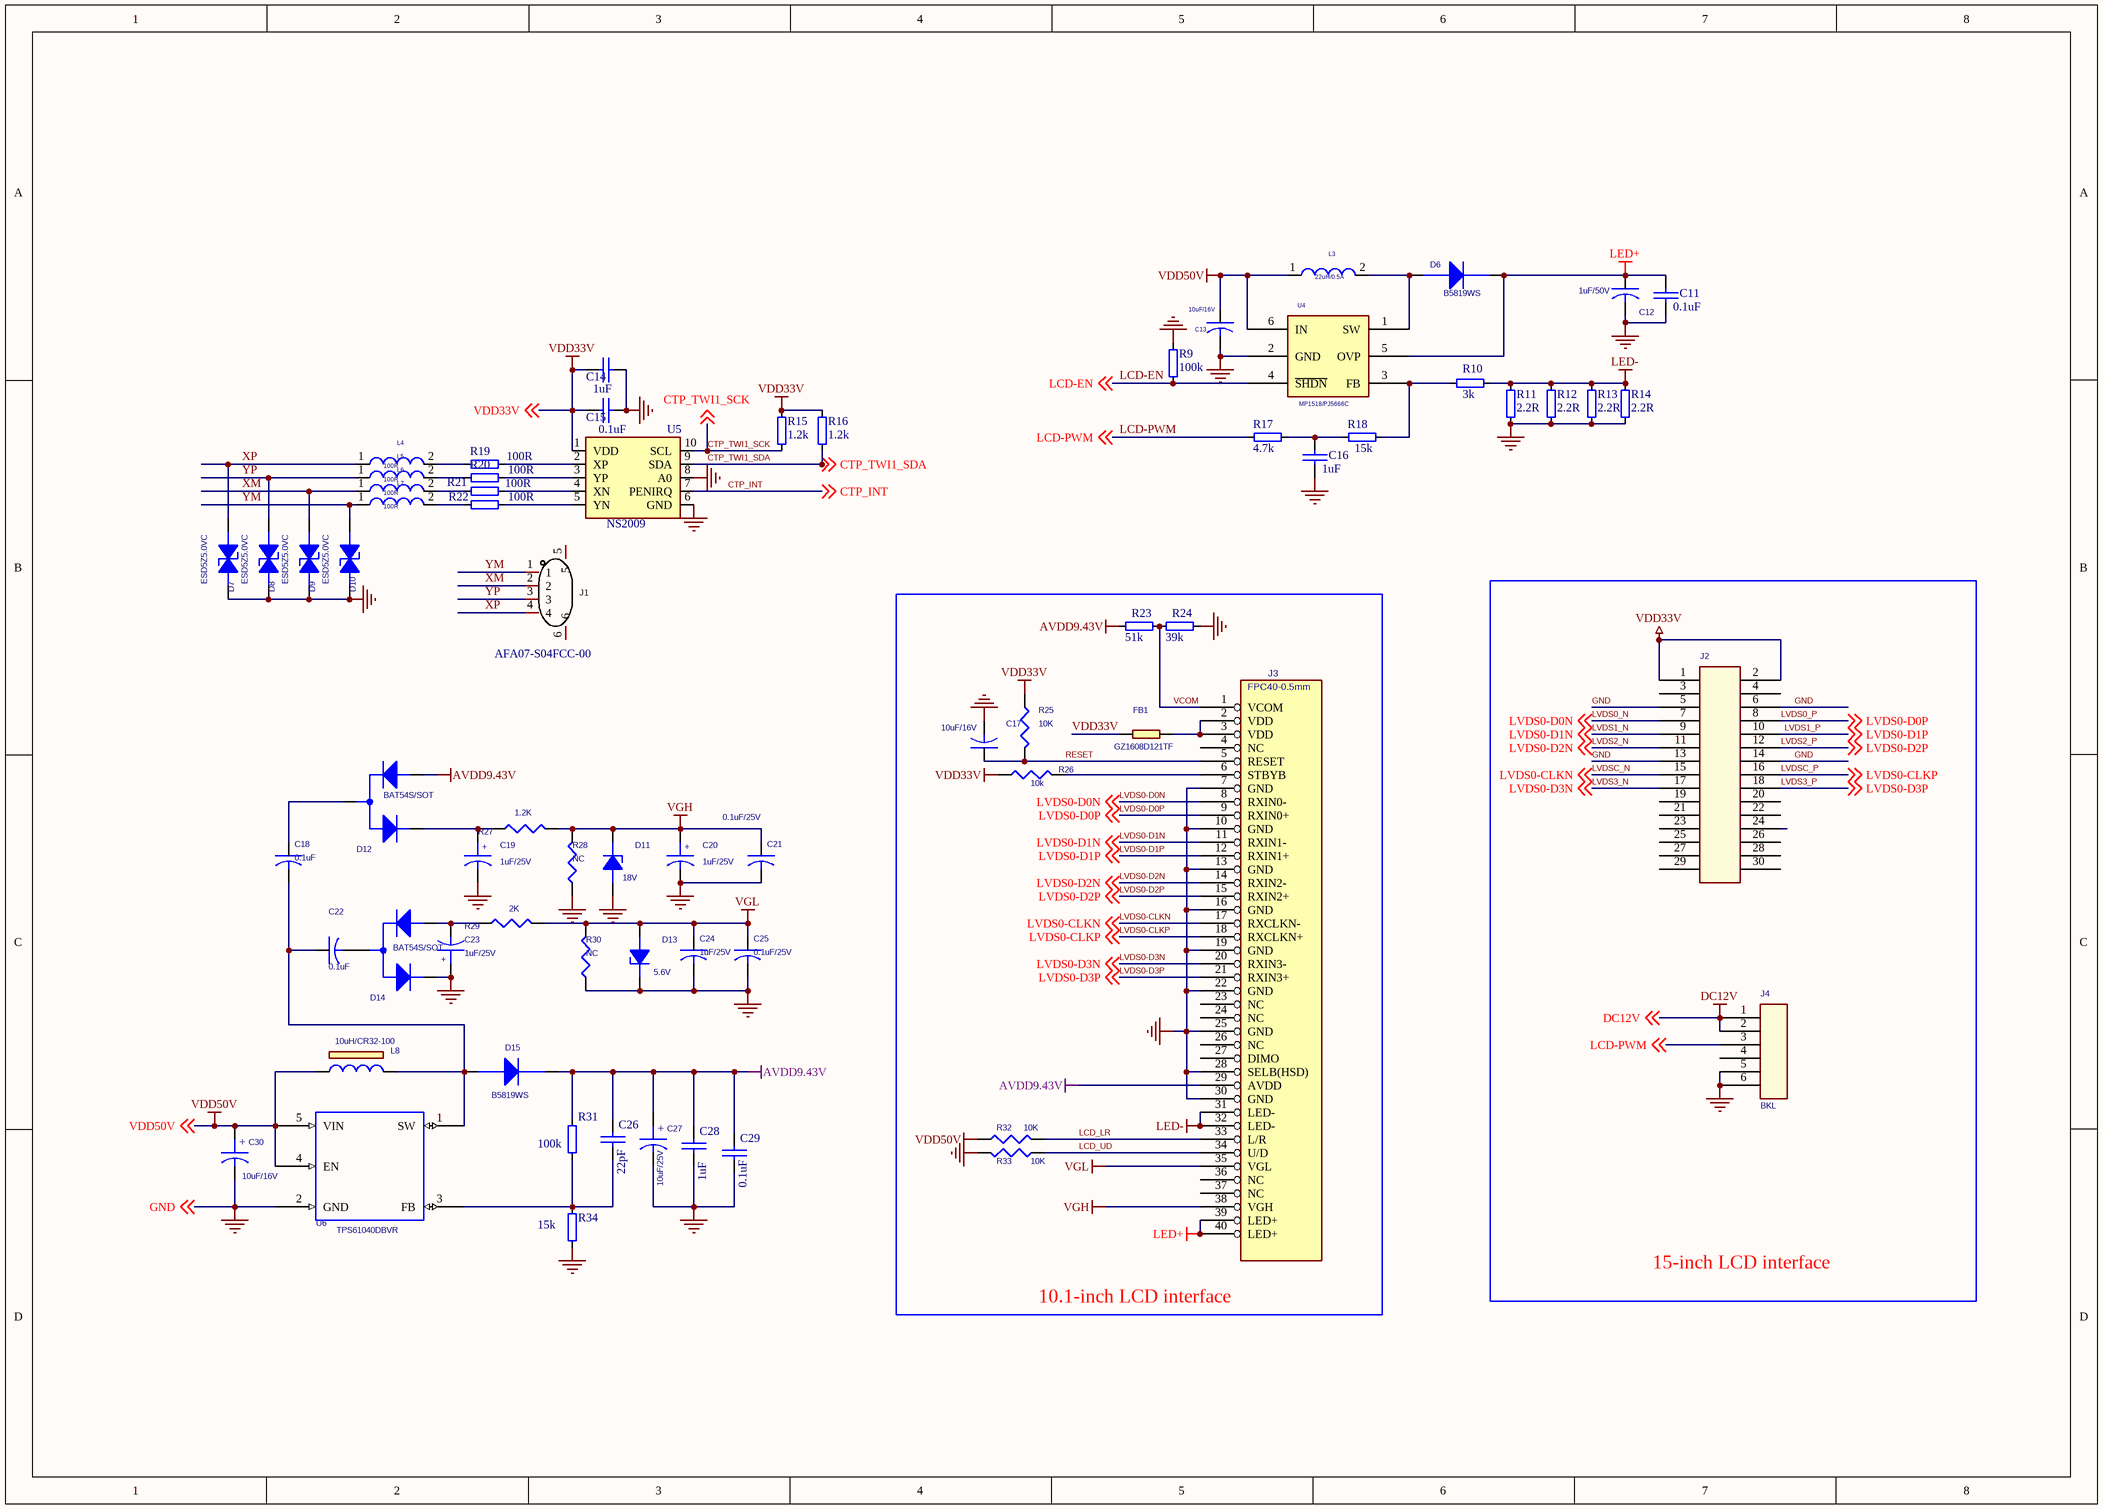
[diagram p0: MISC82162-9.SchDoc]
# Altium schematic sheet MISC82162-9.SchDoc
size A3

## Parts
C11  0.1uF  [0603C]
C12  1uF/50V  [0603C]
C13  10uF/16V  [0603C]
C14  1uF  [0603C]
C15  0.1uF  [0603C]
C16  1uF  [0603C]
C17  10uF/16V  [0603C]
C18  0.1uF  [0603C]
C19  1uF/25V  [C0805]
C20  1uF/25V  [C0805]
C21  0.1uF/25V  [0603C]
C22  0.1uF  [0603C]
C23  1uF/25V  [C0805]
C24  1uF/25V  [0603C]
C25  0.1uF/25V  [0603C]
C26  22pF  [0603C]
C27  10uF/25V  [C0805]
C28  1uF  [0603C]
C29  0.1uF  [0603C]
C30  10uF/16V  [0603C]
D6  B5819WS  [SOD-123]
D7  ESD5Z5.0VC  [SOD-523]
D8  ESD5Z5.0VC  [SOD-523]
D9  ESD5Z5.0VC  [SOD-523]
D10  ESD5Z5.0VC  [SOD-523]
D11  18V  [SOD-123]
D12  BAT54S/SOT  [SOT23]
D13  5.6V  [SOD-123]
D14  BAT54S/SOT  [SOT23]
D15  B5819WS  [SOD-123]
FB1  Part Number: GZ1608D121TF  [CZ0603]  (hidden comment: CZ120)
J1  AFA07-S04FCC-00  [FPC-SMD-1mm4P-RTP]
J2  CON30A  [PH2.0-2X15]  (value not drawn)
J3  FPC40-0.5mm  [FPC40-0.5MM-UP]
J4  BKL  [PH-2.0-6P]
L3  22uH/0.5A  [L-SMD-4*4*1.2]
L4  100R  [L-SMD-4*4*1.2]
L5  100R  [L-SMD-4*4*1.2]
L6  100R  [L-SMD-4*4*1.2]
L7  100R  [L-SMD-4*4*1.2]
L8  10uH/CR32-100  [L-SMD-4*4*1.2]
R9  100k  [0805R]
R10  3k  [0603R]
R11  2.2R  [0805R]
R12  2.2R  [0805R]
R13  2.2R  [0805R]
R14  2.2R  [0805R]
R15  1.2k  [0603R]
R16  1.2k  [0603R]
R17  4.7k  [0603R]
R18  15k  [0603R]
R19  100R  [0603R]
R20  100R  [0603R]
R21  100R  [0603R]
R22  100R  [0603R]
R23  51k  [0603R]
R24  39k  [0603R]
R25  10K  [0603R]
R26  10k  [0603R]
R27  1.2K  [0603R]
R28  NC  [0603R]
R29  2K  [0603R]
R30  NC  [0603R]
R31  100k  [0603R]
R32  10K  [0603R]
R33  10K  [0603R]
R34  15k  [0603R]
U4  MP1518/PJ5666C  [SOT-23-6]
U5  NS2009  [MSOP-10]
U6  TPS61040DBVR  [SOT-23-5]

## Blocks framed on the sheet
10.1-inch LCD interface: C17 FB1 J3 R23-R26 R32 R33
15-inch LCD interface: J2 J4

## Nets
AVDD9.43V: C26.1 C27.1 C28.1 C29.1 D12.1 D15.2(CATHODE) J3.29(AVDD) R23.1 R31.2
DC12V: J4.1 J4.2 ; off-sheet DC12V
GND: C11.2 C12.2 C13.2 C14.2 C15.2 C16.2 C17.2 C19.2 C20.2 C21.2 C23.1 C24.2 C25.2 C27.2 C28.2 C29.2 C30.2 D7.2(CATHODE) D8.2(CATHODE) D9.2(CATHODE) D10.2(CATHODE) D11.1(ANODE) D13.2(CATHODE) D14.2 J2.5 J2.6 J2.13 J2.14 J3.7(GND) J3.10(GND) J3.13(GND) J3.16(GND) J3.19(GND) J3.22(GND) J3.25(GND) J3.28(SELB(HSD)) J3.30(GND) J4.5 J4.6 R9.1 R11.2 R12.2 R13.2 R14.2 R24.2 R28.1 R30.1 R33.2 R34.1 U4.2(GND) U5.6(GND) U5.8(A0) U6.2(GND) ; off-sheet GND
LED+: C11.1 C12.1 D6.2(CATHODE) J3.39(LED+) J3.40(LED+) U4.5(OVP)
LED-: J3.31(LED-) J3.32(LED-) R10.1 R11.1 R12.1 R13.1 R14.1
VDD33V: C14.1 C15.1 FB1.1 J2.1 J2.2 R15.1 R16.1 R25.1 R26.1 U5.1(VDD) ; off-sheet VDD33V
VDD50V: C13.1 C30.1 L3.1 L8.1 R32.1 U4.6(IN) U6.4(EN) U6.5(VIN) ; off-sheet VDD50V
VGH: C20.1 C21.1 D11.2(CATHODE) J3.38(VGH) R27.2 R28.2
VGL: C24.1 C25.1 D13.1(ANODE) J3.35(VGL) R29.2 R30.2
CTP_INT: U5.7(PENIRQ) ; off-sheet CTP_INT
CTP_TWI1_SCK: R15.2 U5.10(SCL) ; off-sheet CTP_TWI1_SCK
CTP_TWI1_SDA: R16.2 U5.9(SDA) ; off-sheet CTP_TWI1_SDA
LCD-EN: R9.2 U4.4(~{SHDN}) ; off-sheet LCD-EN
LCD-PWM: J4.3 R17.2 ; off-sheet LCD-PWM
LCD_LR: J3.33(L/R) R32.2
LCD_UD: J3.34(U/D) R33.1
LVDS0-CLKN: J2.15 J3.17(RXCLKN-) ; off-sheet LVDS0-CLKN  [also labelled LVDSC_N]
LVDS0-CLKP: J2.16 J3.18(RXCLKN+) ; off-sheet LVDS0-CLKP  [also labelled LVDSC_P]
LVDS0-D0N: J2.7 J3.8(RXIN0-) ; off-sheet LVDS0-D0N  [also labelled LVDS0_N]
LVDS0-D0P: J2.8 J3.9(RXIN0+) ; off-sheet LVDS0-D0P  [also labelled LVDS0_P]
LVDS0-D1N: J2.9 J3.11(RXIN1-) ; off-sheet LVDS0-D1N  [also labelled LVDS1_N]
LVDS0-D1P: J2.10 J3.12(RXIN1+) ; off-sheet LVDS0-D1P  [also labelled LVDS1_P]
LVDS0-D2N: J2.11 J3.14(RXIN2-) ; off-sheet LVDS0-D2N  [also labelled LVDS2_N]
LVDS0-D2P: J2.12 J3.15(RXIN2+) ; off-sheet LVDS0-D2P  [also labelled LVDS2_P]
LVDS0-D3N: J2.17 J3.20(RXIN3-) ; off-sheet LVDS0-D3N  [also labelled LVDS3_N]
LVDS0-D3P: J2.18 J3.21(RXIN3+) ; off-sheet LVDS0-D3P  [also labelled LVDS3_P]
RESET: C17.1 J3.5(RESET) R25.2
VCOM: J3.1(VCOM) R23.2 R24.1
XM: D9.1(ANODE) J1.2 L6.1
XP: D7.1(ANODE) J1.4 L4.1
YM: D10.1(ANODE) J1.1 L7.1
YP: D8.1(ANODE) J1.3 L5.1
NetC16_1: C16.1 R17.1 R18.2
NetC18_1: C18.1 D12.3
NetC18_2: C18.2 C22.1 D15.1(ANODE) L8.2 U6.1(SW)
NetC19_1: C19.1 D12.2 R27.1
NetC22_2: C22.2 D14.3
NetC23_2: C23.2 D14.1 R29.1
NetC26_2: C26.2 R31.1 R34.2 U6.3(FB)
NetD6_1: D6.1(ANODE) L3.2 U4.1(SW)
NetFB1_2: FB1.2 J3.2(VDD) J3.3(VDD)
NetJ3_6: J3.6(STBYB) R26.2
NetL4_2: L4.2 R19.1
NetL5_2: L5.2 R20.1
NetL6_2: L6.2 R21.1
NetL7_2: L7.2 R22.1
NetR10_2: R10.2 R18.1 U4.3(FB)
NetR19_2: R19.2 U5.2(XP)
NetR20_2: R20.2 U5.3(YP)
NetR21_2: R21.2 U5.4(XN)
NetR22_2: R22.2 U5.5(YN)

Not connected (* = marked no-connect by the designer): J1 5 6; J2 3 4 19 20 21 22 23 24 25 26 27 28 29 30; J3 4(NC) 23(NC) 24(NC) 26(NC) 27(DIMO) 36(NC) 37(NC); J4 4

## Library data of the parts
C11 C14-C16 C26 C28 C29 = CAP: Capacitor
C12 C17 = C_Dup1
C13 C18 C21 C22 C24 C25 = C
C19 C20 C23 C27 C30 = CAP POL
D6 D15 = BAS21/SOT_1
D7-D10 = 1_1.5KE100A: 1ST PART DESCRIPTION: WILL ESD9B5V Bidirection ESD Protection
D11 D13 = DIODE BREAKDOWN_1
FB1 = FB_1: 180兌(100MHz)_0.05兌_2.0A
J1 = AFC07-S04ECC-00: Manufacturer: JS(钜硕电子); Symbol: FPC 0.5MM 4P Pull type H2.0mm Pick up; Add into BOM: yes; Pitch: 0.5mm; Number of Contacts: 4; Locking Feature: Drawer type; FFC, FCB Thickness: 0.3mm; Name: AFC07-S04ECC-00; Device: AFC07-S04ECC-00; LCSC Part Name: 0.5mm P数:4 抽屉式 上接; Supplier Part: C11082; Manufacturer Part: AFC07-S04ECC-00; Supplier Footprint: SMD,P=0.5mm; JLCPCB Part Class: Extended Part; Supplier: LCSC; Convert to PCB: yes; Mounting Type: Horizontal mount; Contact Type: Top entry; Height Above Board: 2mm
J2 = CON20A_0
J3 = HEADER 20X2_3: Populate: YES
J4 = CON6
L3-L7 = INDUCTOR
L8 = CHOKE TORROID-FERRITE
R9-R20 R22-R24 R31 R34 = RES2
R21 = RES2: Designator: R?
R25 R26 R32 R33 = R_Dup1
R27-R30 = RESISTOR
U4 = PT4110_0
U6 = X9C102/SO_2